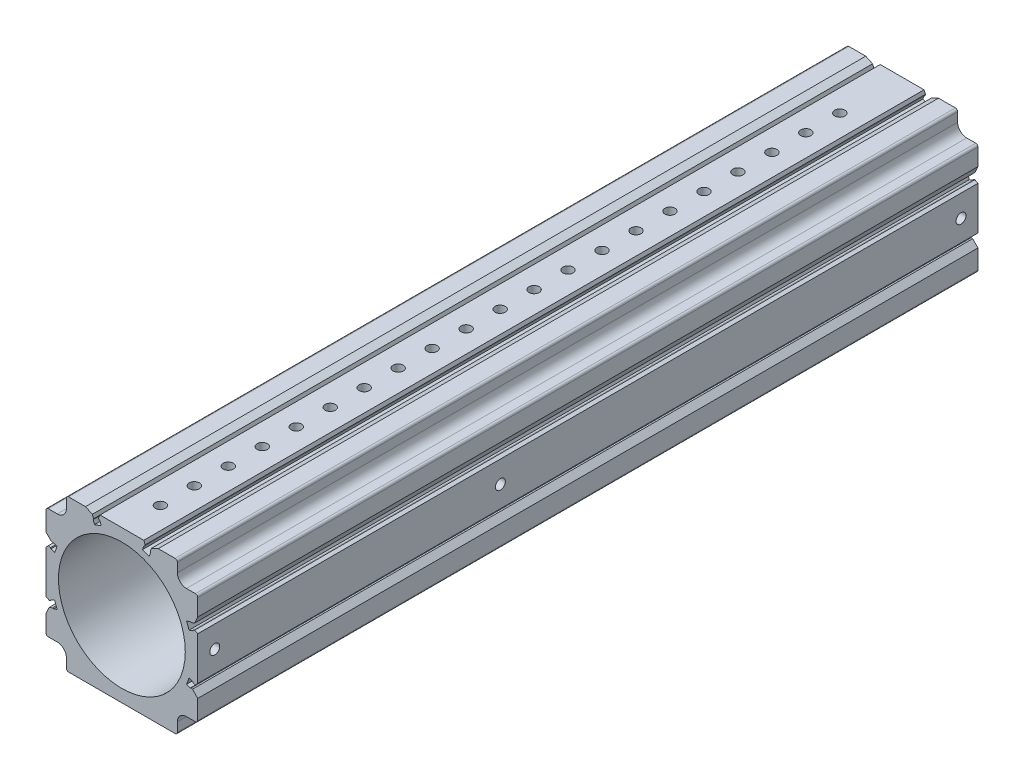
from build123d import *
from OCP.BRepFilletAPI import BRepFilletAPI_MakeChamfer

# Parameters (mm, degrees)
SKETCH1_R                 = 56
BOSS_EXTRUDE1_DEPTH       = 689
SKETCH3_W                 = 24.000744141
SKETCH3_H                 = 31.311653019
CUT_EXTRUDE2_DEPTH        = 696.484723053
FILLET1_R                 = 8
CIRPATTERN1_COUNT         = 4
FILLET1_OF_CIRPATTERN1_R  = 8
LPATTERN1_COUNT           = 21
LPATTERN1_PITCH           = 30
G1_8_TAPPED_HOLE1_D       = 8.8
G1_8_TAPPED_HOLE1_DEPTH   = 22.18
G1_8_TAPPED_HOLE1_TIP     = 2.643786724
FILLET2_R                 = 2
G1_8_TAPPED_HOLE2_D       = 8.8
G1_8_TAPPED_HOLE2_DEPTH   = 22.18
G1_8_TAPPED_HOLE2_TIP     = 2.643786724
CUT_EXTRUDE4_DEPTH        = 696.484723171
BOSS_EXTRUDE3_DEPTH       = 689
CHAMFER2_SIZE             = 3
CHAMFER2_SIZE2            = 2.340618026
CHAMFER3_SIZE             = 3
CHAMFER3_SIZE2            = 5.019471555
CHAMFER2_OF_MIRROR1_SIZE2 = 2.340618026
CHAMFER2_OF_MIRROR1_SIZE  = 3
CHAMFER3_OF_MIRROR1_SIZE2 = 5.019471555
CHAMFER3_OF_MIRROR1_SIZE  = 3
CIRPATTERN13_COUNT        = 4
CIRPATTERN14_COUNT        = 4
MIRROR2_COPY_1_DEPTH      = 696.484723171
MIRROR2_COPY_2_DEPTH      = 696.484723171
BOSS_EXTRUDE4_DEPTH       = 689
CHAMFER4_SIZE             = 3
CHAMFER4_SIZE2            = 2.340618026
CHAMFER4_SIZE2_2          = 5.019471555


with BuildPart() as part:
    # Sketch1 → Boss-Extrude1 (new body)
    with BuildSketch(Plane.XY):
        with BuildLine():
            Line((-44.8, 67), (-36.913248654, 67))
            Line((-36.913248654, 67), (-32.6, 67))
            Line((-32.6, 67), (-32.6, 66.1))
            Line((-32.6, 66.1), (-33.2, 65.5))
            Line((-33.2, 65.5), (-33.2, 62))
            Line((-33.2, 62), (-26.9, 62))
            Line((-26.9, 62), (-26.9, 65.5))
            Line((-26.9, 65.5), (-27.5, 66.1))
            Line((-27.5, 66.1), (-27.5, 67))
            Line((-27.5, 67), (27.5, 67))
            Line((27.5, 67), (27.5, 66.1))
            Line((27.5, 66.1), (26.9, 65.5))
            Line((26.9, 65.5), (26.9, 62))
            Line((26.9, 62), (33.2, 62))
            Line((33.2, 62), (33.2, 65.5))
            Line((33.2, 65.5), (32.6, 66.1))
            Line((32.6, 66.1), (32.6, 67))
            Line((32.6, 67), (36.913248654, 67))
            Line((36.913248654, 67), (44.8, 67))
            Line((44.8, 67), (57, 67))
            ThreePointArc((57, 67), (64.071067812, 64.071067812), (67, 57))
            Line((67, 57), (67, 44.8))
            Line((67, 44.8), (67, 36.913248654))
            Line((67, 36.913248654), (67, 32.6))
            Line((67, 32.6), (66.1, 32.6))
            Line((66.1, 32.6), (65.5, 33.2))
            Line((65.5, 33.2), (62, 33.2))
            Line((62, 33.2), (62, 26.9))
            Line((62, 26.9), (65.5, 26.9))
            Line((65.5, 26.9), (66.1, 27.5))
            Line((66.1, 27.5), (67, 27.5))
            Line((67, 27.5), (67, -27.5))
            Line((67, -27.5), (66.1, -27.5))
            Line((66.1, -27.5), (65.5, -26.9))
            Line((65.5, -26.9), (62, -26.9))
            Line((62, -26.9), (62, -33.2))
            Line((62, -33.2), (65.5, -33.2))
            Line((65.5, -33.2), (66.1, -32.6))
            Line((66.1, -32.6), (67, -32.6))
            Line((67, -32.6), (67, -36.913248654))
            Line((67, -36.913248654), (67, -44.8))
            Line((67, -44.8), (67, -57))
            ThreePointArc((67, -57), (64.071067812, -64.071067812), (57, -67))
            Line((57, -67), (44.8, -67))
            Line((44.8, -67), (36.913248654, -67))
            Line((36.913248654, -67), (-36.913248654, -67))
            Line((-36.913248654, -67), (-44.8, -67))
            Line((-44.8, -67), (-57, -67))
            ThreePointArc((-57, -67), (-64.071067812, -64.071067812), (-67, -57))
            Line((-67, -57), (-67, -44.8))
            Line((-67, -44.8), (-67, -36.913248654))
            Line((-67, -36.913248654), (-67, -32.6))
            Line((-67, -32.6), (-66.1, -32.6))
            Line((-66.1, -32.6), (-65.5, -33.2))
            Line((-65.5, -33.2), (-62, -33.2))
            Line((-62, -33.2), (-62, -26.9))
            Line((-62, -26.9), (-65.5, -26.9))
            Line((-65.5, -26.9), (-66.1, -27.5))
            Line((-66.1, -27.5), (-67, -27.5))
            Line((-67, -27.5), (-67, 27.5))
            Line((-67, 27.5), (-66.1, 27.5))
            Line((-66.1, 27.5), (-65.5, 26.9))
            Line((-65.5, 26.9), (-62, 26.9))
            Line((-62, 26.9), (-62, 33.2))
            Line((-62, 33.2), (-65.5, 33.2))
            Line((-65.5, 33.2), (-66.1, 32.6))
            Line((-66.1, 32.6), (-67, 32.6))
            Line((-67, 32.6), (-67, 36.913248654))
            Line((-67, 36.913248654), (-67, 44.8))
            Line((-67, 44.8), (-67, 57))
            ThreePointArc((-67, 57), (-64.071067812, 64.071067812), (-57, 67))
            Line((-57, 67), (-44.8, 67))
        make_face()
        Circle(SKETCH1_R, mode=Mode.SUBTRACT)
    extrude(amount=BOSS_EXTRUDE1_DEPTH)

    # Sketch3 → Cut-Extrude2 (cut, through all)
    with BuildSketch(Plane.XY.offset(689)):
        with Locations((-61.00037207, 64.65582651)):
            Rectangle(SKETCH3_W, SKETCH3_H)
    cut_extrude2 = extrude(amount=-CUT_EXTRUDE2_DEPTH, mode=Mode.SUBTRACT)

    # Fillet1
    fillet1_edges = [part.edges().sort_by_distance(p)[0] for p in [
        (-49, 49, 344.5),
    ]]
    fillet(fillet1_edges, radius=FILLET1_R)

    # CirPattern1: Cut-Extrude2 ×4 about axis
    cirpattern1_axis = Axis((0, 0, 0), (0, 0, 1))
    for i in range(1, CIRPATTERN1_COUNT):
        add(cut_extrude2.rotate(cirpattern1_axis, i * 360 / CIRPATTERN1_COUNT), mode=Mode.SUBTRACT)

    # Fillet1 of CirPattern1
    fillet1_of_cirpattern1_edges = [part.edges().sort_by_distance(p)[0] for p in [
        (-49, -49, 344.5),
        (49, -49, 344.5),
        (49, 49, 344.5),
    ]]
    fillet(fillet1_of_cirpattern1_edges, radius=FILLET1_OF_CIRPATTERN1_R)

    # Sketch8 → Ø9.0 (9) Diameter Hole1 (revolve, cut)
    with BuildSketch(Plane(origin=(0, 67, 655), x_dir=(0, 0, 1), z_dir=(1, 0, 0))):
        Polygon((0, 0), (0, 22.703872786), (4.5, 20), (4.5, 0), align=None)
    f_9_0_9_diameter_hole1 = revolve(axis=Axis((0, 73.35, 655), (0, -1, 0)), mode=Mode.SUBTRACT)

    # LPattern1: Ø9.0 (9) Diameter Hole1 ×21
    with Locations(*[(0, 0, -i * LPATTERN1_PITCH) for i in range(1, LPATTERN1_COUNT)]):
        add(f_9_0_9_diameter_hole1, mode=Mode.SUBTRACT)

    # G1/8 Tapped Hole1
    with Locations(Plane(origin=(67, 0, 0), x_dir=(0, 0, -1), z_dir=(1, 0, 0))):
        with Locations((-421.8, 0)):
            Hole(G1_8_TAPPED_HOLE1_D / 2, depth=G1_8_TAPPED_HOLE1_DEPTH)
            with Locations((0, 0, -(G1_8_TAPPED_HOLE1_DEPTH + G1_8_TAPPED_HOLE1_TIP / 2))):  # 118° drill point
                Cone(0, G1_8_TAPPED_HOLE1_D / 2, G1_8_TAPPED_HOLE1_TIP, mode=Mode.SUBTRACT)

    # Fillet2
    fillet2_edges = [part.edges().sort_by_distance(p)[0] for p in [
        (-67, 49, 344.5),
        (-49, 67, 344.5),
        (49, 67, 344.5),
        (67, 49, 344.5),
        (67, -49, 344.5),
        (-49, -67, 344.5),
        (49, -67, 344.5),
        (-67, -49, 344.5),
    ]]
    fillet(fillet2_edges, radius=FILLET2_R)

    # G1/8 Tapped Hole2
    with Locations(Plane(origin=(67, 0, 0), x_dir=(0, 0, -1), z_dir=(1, 0, 0))):
        with Locations((-674, 0), (-15, 0)):
            Hole(G1_8_TAPPED_HOLE2_D / 2, depth=G1_8_TAPPED_HOLE2_DEPTH)
            with Locations((0, 0, -(G1_8_TAPPED_HOLE2_DEPTH + G1_8_TAPPED_HOLE2_TIP / 2))):  # 118° drill point
                Cone(0, G1_8_TAPPED_HOLE2_D / 2, G1_8_TAPPED_HOLE2_TIP, mode=Mode.SUBTRACT)

    # Sketch25 → Cut-Extrude4 (cut, through all)
    with BuildSketch(Plane.XY.offset(689)):
        Polygon((-18.245217131, 59.33830594), (-24.165280642, 57.183579037), (-25.362351143, 60.47250321), (-25.003747657, 61.241530868), (-27.490726906, 68.074450198), (-22.69829454, 69.818752929), (-20.211315291, 62.985833599), (-19.442287632, 62.627230113), align=None)
    cut_extrude4 = extrude(amount=-CUT_EXTRUDE4_DEPTH, mode=Mode.SUBTRACT)

    # Sketch26 → Boss-Extrude3 (add, through all)
    with BuildSketch(Plane.XY.offset(689)):
        Polygon((-27.5, 67), (-26.290037253, 64.429630239), (-26.460290585, 61.340748366), (-34.000080984, 61.14617313), (-34.000080984, 67), align=None)
    boss_extrude3 = extrude(amount=-BOSS_EXTRUDE3_DEPTH)

    # Chamfer2
    chamfer2_edges = [part.edges().sort_by_distance(p)[0] for p in [
        (-21.672352376, 67, 344.5),
    ]]
    chamfer2_side = [part.faces().sort_by_distance(p)[0] for p in [
        (-20.941833833, 64.9929168, 344.5),
    ]]
    chamfer(chamfer2_edges, length=CHAMFER2_SIZE, length2=CHAMFER2_SIZE2, reference=chamfer2_side[0])

    # Chamfer3
    chamfer3_edges = [part.edges().sort_by_distance(p)[0] for p in [
        (-27.099659016, 67, 344.5),
    ]]
    chamfer3_side = [part.faces().sort_by_distance(p)[0] for p in [
        (-26.051703336, 64.120765434, 344.5),
    ]]
    chamfer(chamfer3_edges, length=CHAMFER3_SIZE, length2=CHAMFER3_SIZE2, reference=chamfer3_side[0])

    # Mirror1: Cut-Extrude4, Boss-Extrude3 across plane
    add(cut_extrude4.mirror(Plane(origin=(0, 0, 0), x_dir=(0, 0, 1), z_dir=(1, 0, 0))), mode=Mode.SUBTRACT)
    add(boss_extrude3.mirror(Plane(origin=(0, 0, 0), x_dir=(0, 0, 1), z_dir=(1, 0, 0))))

    # Chamfer2 of Mirror1
    chamfer2_of_mirror1_edges = [part.edges().sort_by_distance(p)[0] for p in [
        (21.672352376, 67, 344.5),
    ]]
    chamfer(chamfer2_of_mirror1_edges, length=CHAMFER2_OF_MIRROR1_SIZE, length2=CHAMFER2_OF_MIRROR1_SIZE2)

    # Chamfer3 of Mirror1
    chamfer3_of_mirror1_edges = [part.edges().sort_by_distance(p)[0] for p in [
        (27.099659016, 67, 344.5),
    ]]
    chamfer(chamfer3_of_mirror1_edges, length=CHAMFER3_OF_MIRROR1_SIZE, length2=CHAMFER3_OF_MIRROR1_SIZE2)

    # CirPattern13: Cut-Extrude4 ×4 about axis, 1 skipped
    cirpattern13_axis = Axis((0, 0, 0), (0, 0, 1))
    add([cut_extrude4.rotate(cirpattern13_axis, i * 360 / CIRPATTERN13_COUNT) for i in range(1, CIRPATTERN13_COUNT) if i not in (2,)], mode=Mode.SUBTRACT)

    # CirPattern14: Boss-Extrude3 ×4 about axis, 1 skipped
    cirpattern14_axis = Axis((0, 0, 689), (0, 0, -1))
    add([boss_extrude3.rotate(cirpattern14_axis, i * 360 / CIRPATTERN14_COUNT) for i in range(1, CIRPATTERN14_COUNT) if i not in (2,)])

    # Mirror2: Cut-Extrude4 across plane
    add(cut_extrude4.mirror(Plane.ZX), mode=Mode.SUBTRACT)

    # Mirror2 copy 1 sketch → Mirror2 copy 1 (cut, through all)
    with BuildSketch(Plane(origin=(0, 0, 689), x_dir=(0, -1, 0), z_dir=(0, 0, 1))):
        Polygon((-18.245217131, -59.33830594), (-24.165280642, -57.183579037), (-25.362351143, -60.47250321), (-25.003747657, -61.241530868), (-27.490726906, -68.074450198), (-22.69829454, -69.818752929), (-20.211315291, -62.985833599), (-19.442287632, -62.627230113), align=None)
    extrude(amount=-MIRROR2_COPY_1_DEPTH, mode=Mode.SUBTRACT)

    # Mirror2 copy 2 sketch → Mirror2 copy 2 (cut, through all)
    with BuildSketch(Plane(origin=(0, 0, 689), x_dir=(0, 1, 0), z_dir=(0, 0, 1))):
        Polygon((-18.245217131, -59.33830594), (-24.165280642, -57.183579037), (-25.362351143, -60.47250321), (-25.003747657, -61.241530868), (-27.490726906, -68.074450198), (-22.69829454, -69.818752929), (-20.211315291, -62.985833599), (-19.442287632, -62.627230113), align=None)
    extrude(amount=-MIRROR2_COPY_2_DEPTH, mode=Mode.SUBTRACT)

    # Sketch28 → Boss-Extrude4 (add, through all)
    with BuildSketch(Plane.XY.offset(689)):
        Polygon((-27.099659016, -67), (-21.672352376, -67), (-15.195943719, -57.916615682), (-28.958307841, -52.946873083), align=None)
        Polygon((-67, 27.5), (-67, 32.6), (-62.005583505, 35.167109027), (-60.064602607, 33.164833995), (-60.766437336, 26.614322888), (-64.028289916, 26.614322888), (-65.677432045, 26.791015241), align=None)
        Polygon((67, -27.5), (67, -32.6), (64.418272864, -34.192896025), (60.864105342, -33.812095479), (60.640482132, -29.234927503), (60.919197603, -26.633561815), (64.751432098, -26.446333253), (66.168921553, -27.078779421), align=None)
    extrude(amount=-BOSS_EXTRUDE4_DEPTH)

    # Chamfer4: one chamfer whose edges measure the first distance from different faces: ONE call of the kernel's chamfer builder (chamfer() names one face for all edges)
    chamfer4_edges_1 = [part.edges().sort_by_distance(p)[0] for p in [
        (-67, -21.672352376, 344.5),
    ]]
    chamfer4_side_1 = [part.faces().sort_by_distance(p)[0] for p in [
        (-64.9929168, -20.941833833, 344.5),
    ]]
    chamfer4_edges_2 = [part.edges().sort_by_distance(p)[0] for p in [
        (-67, -27.099659016, 344.5),
    ]]
    chamfer4_side_2 = [part.faces().sort_by_distance(p)[0] for p in [
        (-64.120765434, -26.051703336, 344.5),
    ]]
    chamfer4_edges_3 = [part.edges().sort_by_distance(p)[0] for p in [
        (67, 21.672352376, 344.5),
    ]]
    chamfer4_side_3 = [part.faces().sort_by_distance(p)[0] for p in [
        (64.9929168, 20.941833833, 344.5),
    ]]
    chamfer4_edges_4 = [part.edges().sort_by_distance(p)[0] for p in [
        (67, 27.099659016, 344.5),
    ]]
    chamfer4_side_4 = [part.faces().sort_by_distance(p)[0] for p in [
        (64.120765434, 26.051703336, 344.5),
    ]]
    chamfer4_edges_5 = [part.edges().sort_by_distance(p)[0] for p in [
        (-67, 27.099659016, 344.5),
    ]]
    chamfer4_side_5 = [part.faces().sort_by_distance(p)[0] for p in [
        (-67, 37.049829508, 344.5),
    ]]
    chamfer4_edges_6 = [part.edges().sort_by_distance(p)[0] for p in [
        (-67, 21.672352376, 344.5),
    ]]
    chamfer4_side_6 = [part.faces().sort_by_distance(p)[0] for p in [
        (-67, 0, 344.5),
    ]]
    chamfer4_edges_7 = [part.edges().sort_by_distance(p)[0] for p in [
        (67, -27.099659016, 344.5),
    ]]
    chamfer4_side_7 = [part.faces().sort_by_distance(p)[0] for p in [
        (67, -37.049829508, 344.5),
    ]]
    chamfer4_edges_8 = [part.edges().sort_by_distance(p)[0] for p in [
        (67, -21.672352376, 344.5),
    ]]
    chamfer4_side_8 = [part.faces().sort_by_distance(p)[0] for p in [
        (67, 0, 344.341605169),
    ]]
    chamfer4 = BRepFilletAPI_MakeChamfer(part.part.solid().wrapped)
    for e in chamfer4_edges_1:
        chamfer4.Add(CHAMFER4_SIZE, CHAMFER4_SIZE2, e.wrapped, chamfer4_side_1[0].wrapped)  # the first distance lies on this face
    for e in chamfer4_edges_2:
        chamfer4.Add(CHAMFER4_SIZE, CHAMFER4_SIZE2_2, e.wrapped, chamfer4_side_2[0].wrapped)  # the first distance lies on this face
    for e in chamfer4_edges_3:
        chamfer4.Add(CHAMFER4_SIZE, CHAMFER4_SIZE2, e.wrapped, chamfer4_side_3[0].wrapped)  # the first distance lies on this face
    for e in chamfer4_edges_4:
        chamfer4.Add(CHAMFER4_SIZE, CHAMFER4_SIZE2_2, e.wrapped, chamfer4_side_4[0].wrapped)  # the first distance lies on this face
    for e in chamfer4_edges_5:
        chamfer4.Add(CHAMFER4_SIZE, CHAMFER4_SIZE2_2, e.wrapped, chamfer4_side_5[0].wrapped)  # the first distance lies on this face
    for e in chamfer4_edges_6:
        chamfer4.Add(CHAMFER4_SIZE, CHAMFER4_SIZE2, e.wrapped, chamfer4_side_6[0].wrapped)  # the first distance lies on this face
    for e in chamfer4_edges_7:
        chamfer4.Add(CHAMFER4_SIZE, CHAMFER4_SIZE2_2, e.wrapped, chamfer4_side_7[0].wrapped)  # the first distance lies on this face
    for e in chamfer4_edges_8:
        chamfer4.Add(CHAMFER4_SIZE, CHAMFER4_SIZE2, e.wrapped, chamfer4_side_8[0].wrapped)  # the first distance lies on this face
    add(Compound.cast(chamfer4.Shape()), mode=Mode.REPLACE)


solid = part.part
